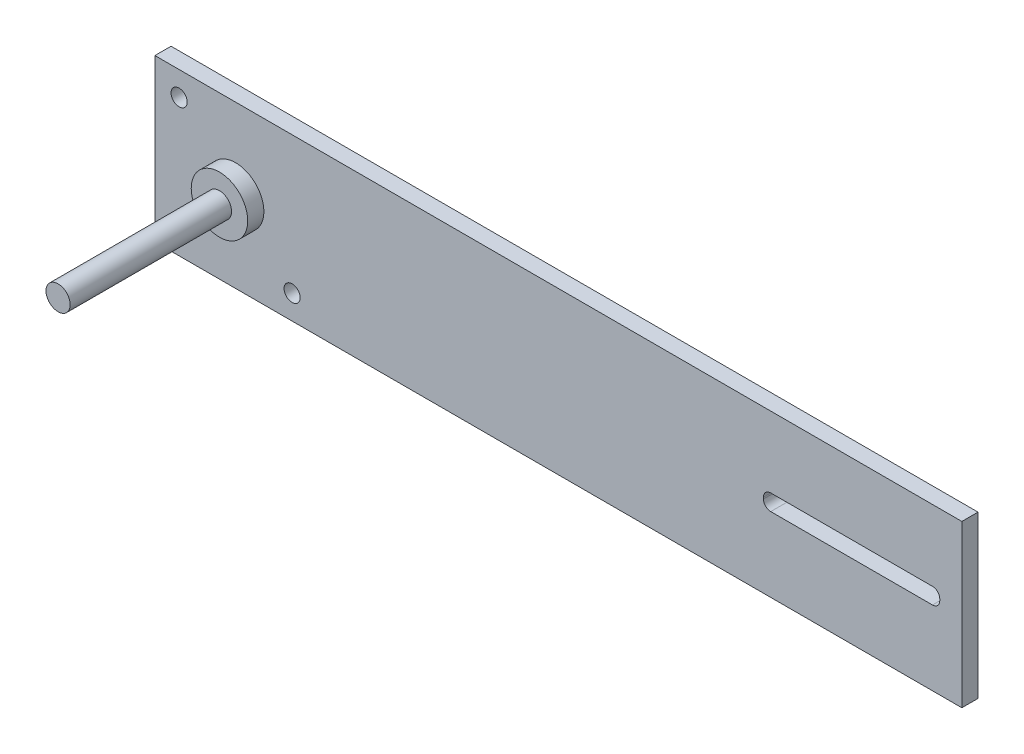
from build123d import *

# Parameters (mm, degrees)
SKETCH1_W           = 500
SKETCH1_H           = 100
BOSS_EXTRUDE1_DEPTH = 10
CUT_EXTRUDE1_DEPTH  = 60
SKETCH4_R           = 5
CUT_EXTRUDE2_DEPTH  = 60
SKETCH2_R           = 17.5
BOSS_EXTRUDE2_DEPTH = 60
CUT_EXTRUDE3_START  = -50
SKETCH5_R           = 17.5
SKETCH5_R_2         = 7.5
CUT_EXTRUDE3_DEPTH  = 50
SKETCH6_R           = 7.5
BOSS_EXTRUDE3_DEPTH = 50


with BuildPart() as part:
    # Sketch1 → Boss-Extrude1 (new body)
    with BuildSketch(Plane.XY):
        Rectangle(SKETCH1_W, SKETCH1_H)
    extrude(amount=BOSS_EXTRUDE1_DEPTH)

    # Sketch3 → Cut-Extrude1 (cut)
    with BuildSketch(Plane.XY.offset(10)):
        with BuildLine():
            Line((231.804981109, -3.932202525), (131.558181165, -3.932202525))
            ThreePointArc((131.558181165, -3.932202525), (128.376200649, -2.614183041), (127.058181165, 0.567797475))
            Line((127.058181165, 0.567797475), (127.058181165, 1.567797475))
            ThreePointArc((127.058181165, 1.567797475), (128.376200649, 4.74977799), (131.558181165, 6.067797475))
            Line((131.558181165, 6.067797475), (231.804981109, 6.067797475))
            ThreePointArc((231.804981109, 6.067797475), (234.986961624, 4.74977799), (236.304981109, 1.567797475))
            Line((236.304981109, 1.567797475), (236.304981109, 0.567797475))
            ThreePointArc((236.304981109, 0.567797475), (234.986961624, -2.614183041), (231.804981109, -3.932202525))
        make_face()
    extrude(amount=-CUT_EXTRUDE1_DEPTH, mode=Mode.SUBTRACT)

    # Sketch4 → Cut-Extrude2 (cut)
    with BuildSketch(Plane.XY.offset(10)):
        with Locations((-235, 35)):
            Circle(SKETCH4_R)
        with Locations((-165, -35)):
            Circle(SKETCH4_R)
    extrude(amount=-CUT_EXTRUDE2_DEPTH, mode=Mode.SUBTRACT)

    # Sketch2 → Boss-Extrude2 (add)
    with BuildSketch(Plane.XY.offset(10)):
        with Locations(Location((-200, 0, 0), (0, 0, 180))):
            Circle(SKETCH2_R)
    extrude(amount=BOSS_EXTRUDE2_DEPTH)

    # Sketch5 → Cut-Extrude3 (cut)
    with BuildSketch(Plane.XY.offset(70).offset(CUT_EXTRUDE3_START)):
        with Locations(Location((-200, 0, 0), (0, 0, 180))):
            Circle(SKETCH5_R)
        with Locations((-200, 0)):
            Circle(SKETCH5_R_2, mode=Mode.SUBTRACT)
    extrude(amount=CUT_EXTRUDE3_DEPTH, mode=Mode.SUBTRACT)

    # Sketch6 → Boss-Extrude3 (add)
    with BuildSketch(Plane.XY.offset(70)):
        with Locations((-200, 0)):
            Circle(SKETCH6_R)
    extrude(amount=BOSS_EXTRUDE3_DEPTH)


solid = part.part
